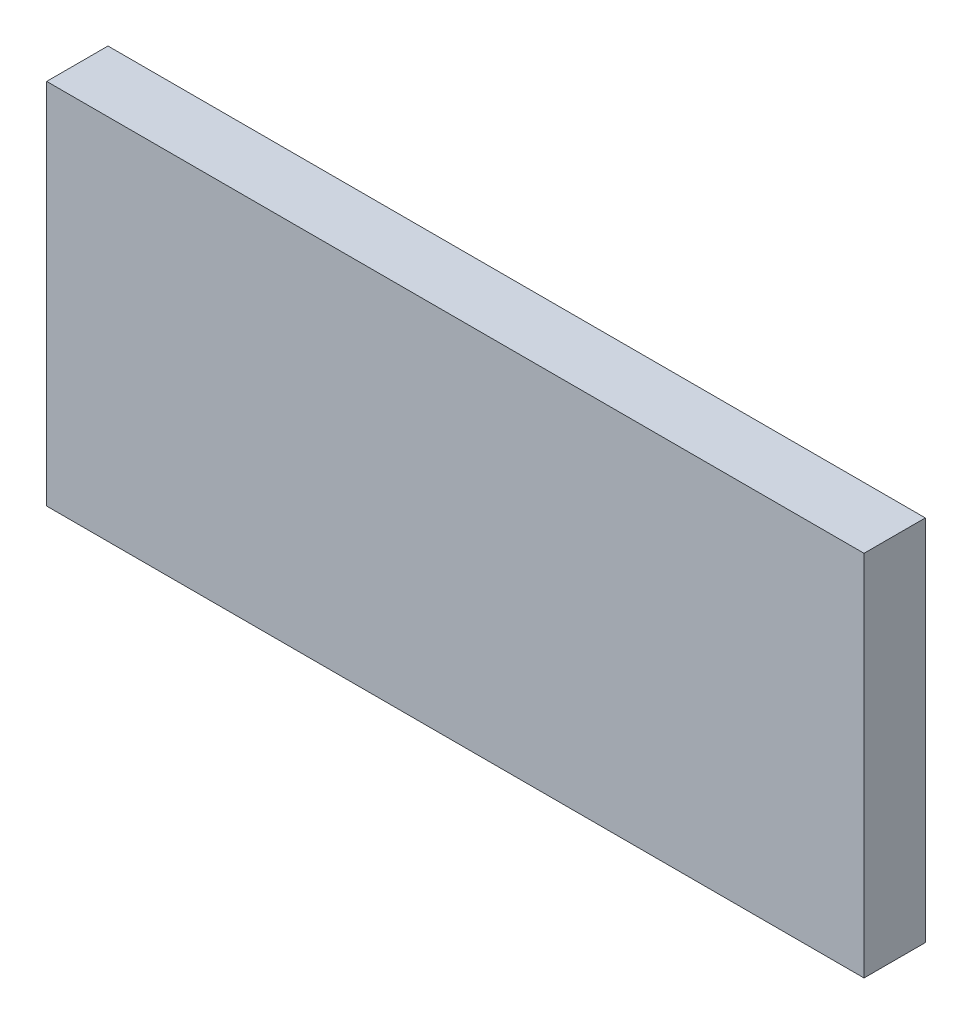
SolidWorks part; units mm, degrees
material "Q235-A"
ref_plane "Front Plane" through (0, 0, 0) normal (0, 0, 1) x (1, 0, 0)
ref_plane "Top Plane" through (0, 0, 0) normal (0, 1, 0) x (1, 0, 0)
ref_plane "Right Plane" through (0, 0, 0) normal (1, 0, 0) x (0, 0, -1)
sketch "Sketch1" plane through (0, 0, 0) normal (0, 0, 1) x (1, 0, 0)
  line L1 (100, -45) -> (-100, -45)
  line L2 (100, -45) -> (100, 45)
  line L3 (100, 45) -> (-100, 45)
  line L4 (-100, -45) -> (-100, 45)
  line L5 (100, -45) -> (-100, 45) construction
  line L6 (100, 45) -> (-100, -45) construction
  point P0 (0, 0)
  dimension "D1" = 90
  dimension "D2" = 200
extrude "Boss-Extrude1" add sketch "Sketch1" along normal mid plane 15
